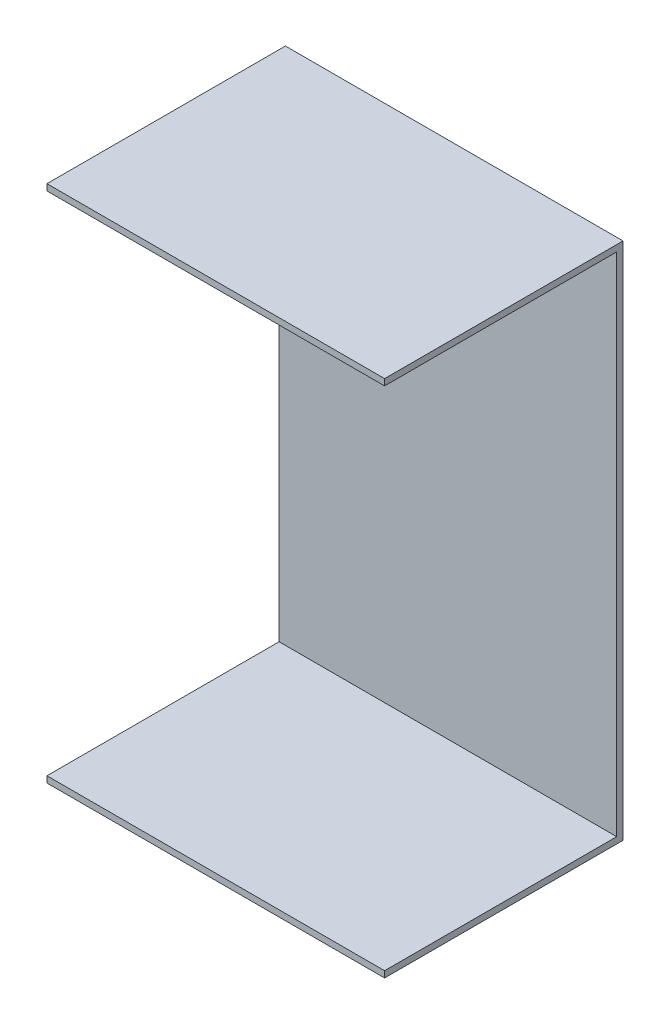
from build123d import *

# Parameters (mm, degrees)
SKETCH1_W           = 160
SKETCH1_H           = 246
BOSS_EXTRUDE1_DEPTH = 3
SKETCH2_W           = 160
SKETCH2_H           = 3
BOSS_EXTRUDE2_DEPTH = 110


with BuildPart() as part:
    # Sketch1 → Boss-Extrude1 (new body)
    with BuildSketch(Plane.XY):
        Rectangle(SKETCH1_W, SKETCH1_H)
    extrude(amount=BOSS_EXTRUDE1_DEPTH)

    # Sketch2 → Boss-Extrude2 (add)
    with BuildSketch(Plane.XY.offset(3)):
        with Locations((0, 121.5)):
            Rectangle(SKETCH2_W, SKETCH2_H)
        with Locations((0, -121.5)):
            Rectangle(SKETCH2_W, SKETCH2_H)
    extrude(amount=BOSS_EXTRUDE2_DEPTH)


solid = part.part
